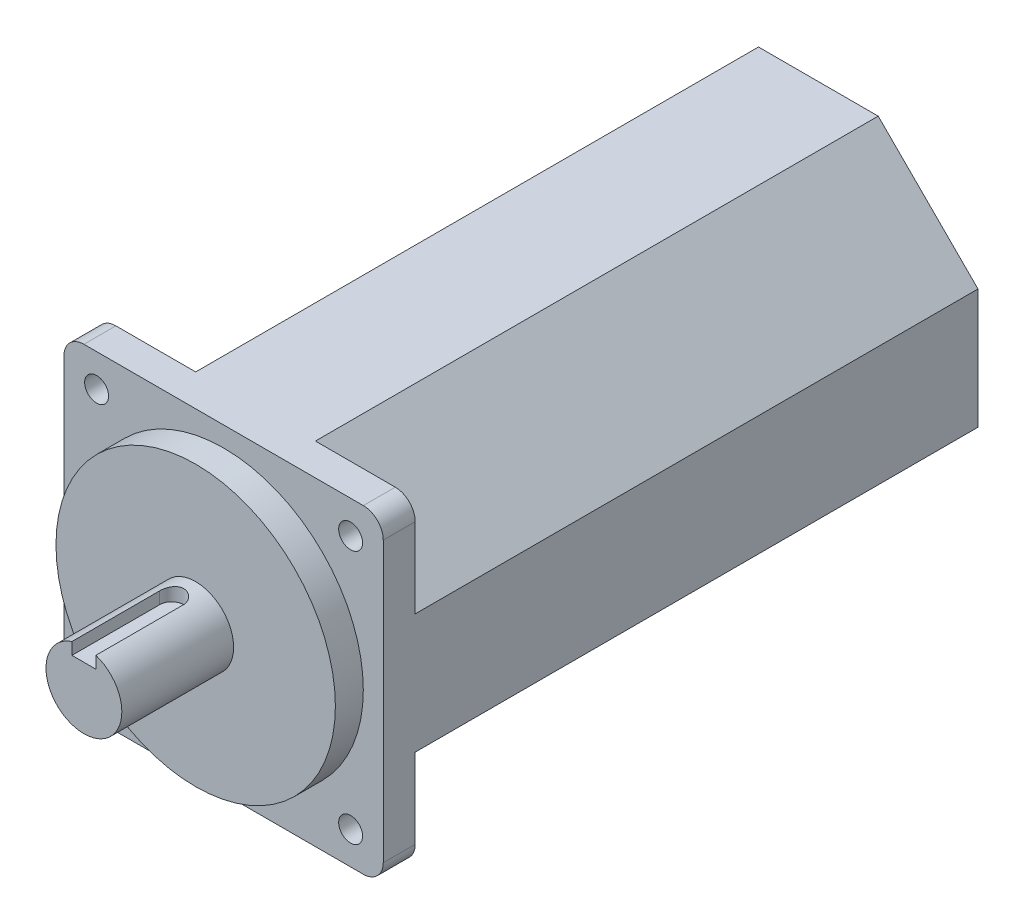
from build123d import *

# Parameters (mm, degrees)
EXTRUDE_1_DEPTH     = 149
SKETCH_2_R          = 35
EXTRUDE_2_DEPTH     = 7
SKETCH_4_W          = 80
SKETCH_4_H          = 80
EXTRUDE_3_DEPTH     = 8
SKETCH_5_R          = 3
CUT_EXTRUDE_1_DEPTH = 8
FILLET_1_R          = 5
SKETCH_6_R          = 9.5
EXTRUDE_4_DEPTH     = 28
SKETCH_7_W          = 6
SKETCH_7_H          = 7.374792238
EXTRUDE_5_DEPTH     = 22
SKETCH_8_R          = 3
CUT_EXTRUDE_2_DEPTH = 34


with BuildPart() as part:
    # 草图1 → 凸台-拉伸1 (new body)
    with BuildSketch(Plane.XY):
        Polygon((25, 80), (0, 55), (0, 25), (25, 0), (55, 0), (80, 25), (80, 55), (55, 80), align=None)
    extrude(amount=EXTRUDE_1_DEPTH)

    # 草图2 → 凸台-拉伸2 (add)
    with BuildSketch(Plane.XY.offset(149)):
        with Locations((40, 40)):
            Circle(SKETCH_2_R)
    extrude(amount=EXTRUDE_2_DEPTH)

    # 草图4 → 凸台-拉伸3 (add)
    with BuildSketch(Plane.XY.offset(149)):
        with Locations((40, 40)):
            Rectangle(SKETCH_4_W, SKETCH_4_H)
    extrude(amount=-EXTRUDE_3_DEPTH)

    # 草图5 → 切除-拉伸1 (cut)
    with BuildSketch(Plane.XY.offset(149)):
        with Locations((8.180194847, 71.819805153)):
            Circle(SKETCH_5_R)
        with Locations((71.819805153, 71.819805153)):
            Circle(SKETCH_5_R)
        with Locations((71.819805153, 8.180194847)):
            Circle(SKETCH_5_R)
        with Locations((8.180194847, 8.180194847)):
            Circle(SKETCH_5_R)
    extrude(amount=-CUT_EXTRUDE_1_DEPTH, mode=Mode.SUBTRACT)

    # 圆角1
    fillet_1_edges = [part.edges().sort_by_distance(p)[0] for p in [
        (0, 0, 145),
        (80, 0, 145),
        (0, 80, 145),
        (80, 80, 145),
    ]]
    fillet(fillet_1_edges, radius=FILLET_1_R)

    # 草图6 → 凸台-拉伸4 (add)
    with BuildSketch(Plane.XY.offset(156)):
        with Locations((40, 40)):
            Circle(SKETCH_6_R)
    extrude(amount=EXTRUDE_4_DEPTH)


with BuildPart() as body_2:
    # 草图7 → 凸台-拉伸5 (new body)
    with BuildSketch(Plane.XY.offset(184)):
        with Locations((40, 49.687396119)):
            Rectangle(SKETCH_7_W, SKETCH_7_H)
    extrude(amount=-EXTRUDE_5_DEPTH)


with BuildPart() as part_1:
    add(part.part)

    # Combine 1: cut body 2
    add(body_2.part, mode=Mode.SUBTRACT)

    # 草图8 → 切除-拉伸2 (cut)
    with BuildSketch(Plane(origin=(0, 80, 0), x_dir=(1, 0, 0), z_dir=(0, 1, 0))):
        with Locations((40, -162)):
            Circle(SKETCH_8_R)
    extrude(amount=-CUT_EXTRUDE_2_DEPTH, mode=Mode.SUBTRACT)


solid = part_1.part
